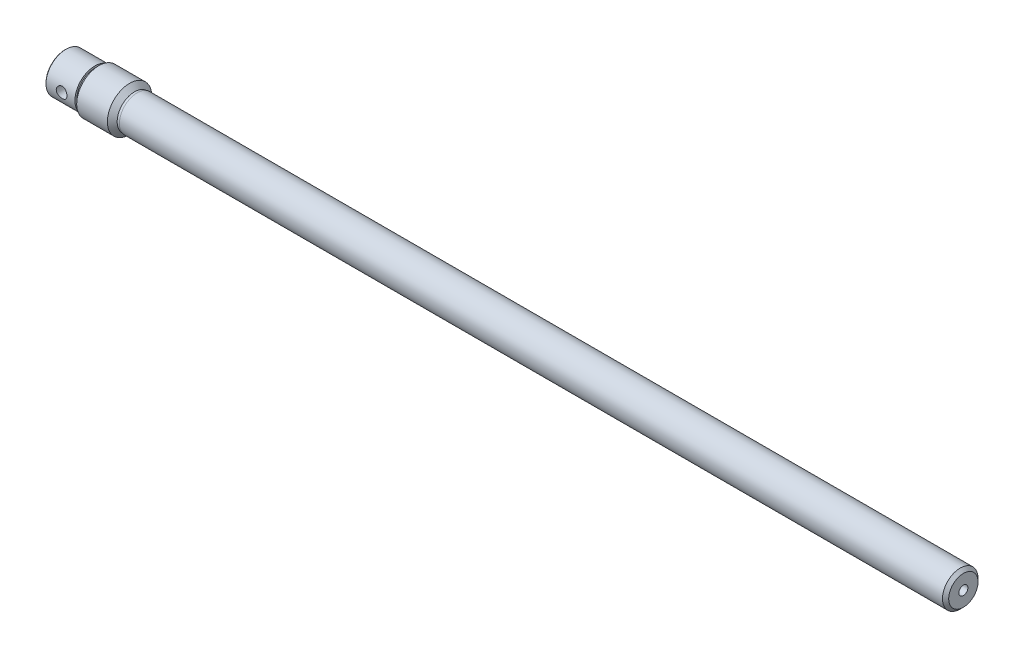
from build123d import *

# Parameters (mm, degrees)
CHAMFER1_SIZE          = 3.5
CHAMFER2_SIZE          = 1
SKETCH2_R              = 6
CUT_EXTRUDE1_DEPTH     = 50
M12_TAPPED_HOLE1_D     = 10.2
M12_TAPPED_HOLE1_DEPTH = 23.25
M12_TAPPED_HOLE1_TIP   = 3.064389157


with BuildPart() as part:
    # Sketch1 → Revolve1 (revolve)
    with BuildSketch(Plane.XY, mode=Mode.PRIVATE) as revolve1_sk:
        Polygon((81, 19.5), (78, 19.5), (72.5, 25), (38, 25), (38, 22.5), (38, 20.3), (33.5, 20.3), (33.5, 22.5), (0, 22.5), (0, 0), (38, 0), (78, 0), (81, 0), (1010, 0), (1010, 20), (81, 20), align=None)
    revolve(revolve1_sk.sketch.rotate(Axis((38, 0, 0), (1, 0, 0)), 90), axis=Axis((38, 0, 0), (1, 0, 0)))

    # Chamfer1
    chamfer1_edges = [part.edges().sort_by_distance(p)[0] for p in [
        (1010, 0, -20),
    ]]
    chamfer(chamfer1_edges, length=CHAMFER1_SIZE)

    # Chamfer2
    chamfer2_edges = [part.edges().sort_by_distance(p)[0] for p in [
        (0, 0, -22.5),
    ]]
    chamfer(chamfer2_edges, length=CHAMFER2_SIZE)

    # Sketch2 → Cut-Extrude1 (cut, symmetric)
    with BuildSketch(Plane.XY):
        with Locations((18.5, 0)):
            Circle(SKETCH2_R)
    extrude(amount=CUT_EXTRUDE1_DEPTH, both=True, mode=Mode.SUBTRACT)

    # M12 Tapped Hole1
    with Locations(Plane(origin=(1010, 0, 0), x_dir=(0, 0, -1), z_dir=(1, 0, 0))):
        with Locations((0, 0)):
            Hole(M12_TAPPED_HOLE1_D / 2, depth=M12_TAPPED_HOLE1_DEPTH)
            with Locations((0, 0, -(M12_TAPPED_HOLE1_DEPTH + M12_TAPPED_HOLE1_TIP / 2))):  # 118° drill point
                Cone(0, M12_TAPPED_HOLE1_D / 2, M12_TAPPED_HOLE1_TIP, mode=Mode.SUBTRACT)


solid = part.part
